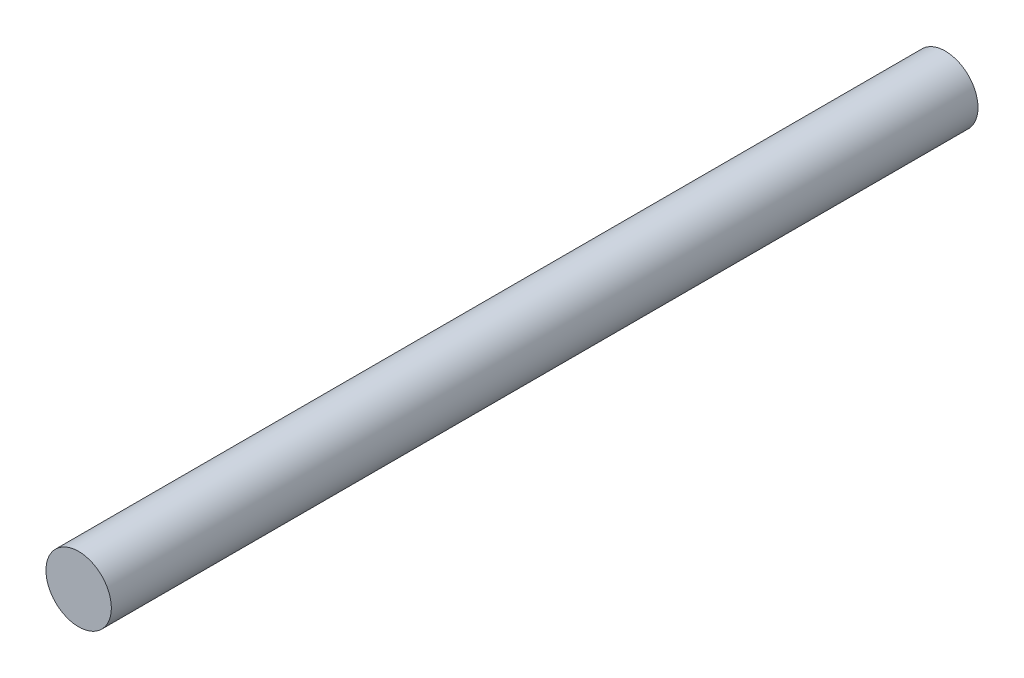
SolidWorks part; units mm, degrees
ref_plane "前视基准面" through (0, 0, 0) normal (0, 0, 1) x (1, 0, 0)
ref_plane "上视基准面" through (0, 0, 0) normal (0, 1, 0) x (1, 0, 0)
ref_plane "右视基准面" through (0, 0, 0) normal (1, 0, 0) x (0, 0, -1)
sketch "草图1" plane through (0, 0, 0) normal (0, 0, 1) x (1, 0, 0)
  circle A0 centre (0, 0) radius 10
  dimension "D1" = 20
extrude "凸台-拉伸1" add sketch "草图1" along normal blind 265
